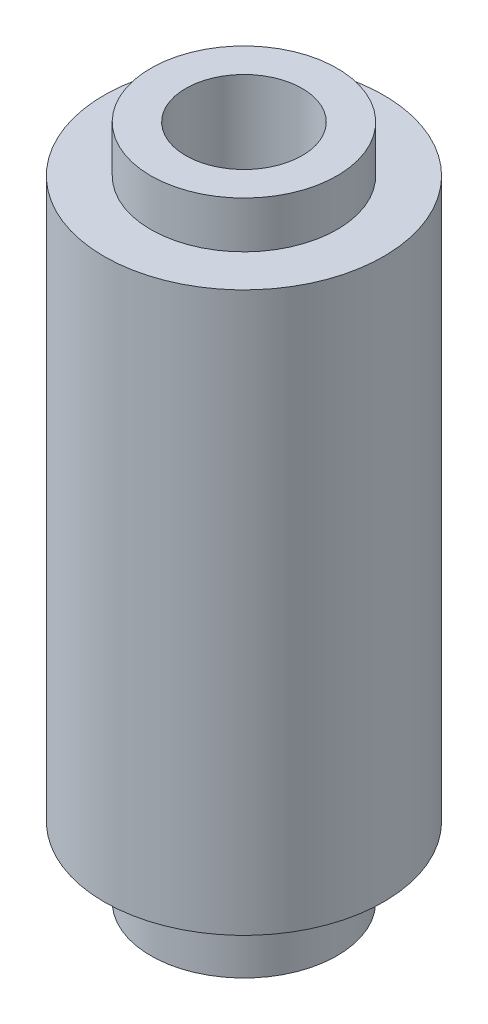
SolidWorks part; units mm, degrees
ref_plane "Front plane" through (0, 0, 0) normal (0, 0, 1) x (1, 0, 0)
ref_plane "Top plane" through (0, 0, 0) normal (0, 1, 0) x (1, 0, 0)
ref_plane "Right plane" through (0, 0, 0) normal (1, 0, 0) x (0, 0, -1)
other "Configuration Table"
sketch "Sketch 2" plane through (0, 0, 0) normal (0, 1, 0) x (1, 0, 0)
  circle A0 centre (0, 0) radius 3
  dimension "D1" = 6
extrude "Boss-Extrude 1" add sketch "Sketch 2" along normal blind 12
sketch "Sketch 3" plane through (0, 12, 0) normal (0, 1, 0) x (1, 0, 0)
  circle A0 centre (0, 0) radius 2
  dimension "D1" = 4
extrude "Boss-Extrude 2" add sketch "Sketch 3" along normal blind 1
sketch "Sketch 4" plane through (0, 0, 0) normal (0, -1, 0) x (-1, 0, 0)
  circle A0 centre (0, 0) radius 2
extrude "Boss-Extrude 3" add sketch "Sketch 4" along normal blind 1.5
sketch "Sketch 5" plane through (0, 13, 0) normal (0, 1, 0) x (1, 0, 0)
  circle A0 centre (0, 0) radius 1.25
  dimension "D1" = 2.5
extrude "Cut-Extrude 1" cut sketch "Sketch 5" against normal blind 6
sketch "Sketch 6" plane through (0, 7, 0) normal (0, 1, 0) x (1, 0, 0)
  circle A0 centre (0, 0) radius 1.5
  dimension "D1" = 3
extrude "Cut-Extrude 2" cut sketch "Sketch 6" against normal blind 2.5
sketch "Sketch 7" plane through (0, -1.5, 0) normal (0, -1, 0) x (-1, 0, 0)
  line L16 (-0.9741, 1.1407) -> (-1.3859, -0.5739)
  line L17 (-1.3859, -0.5739) -> (0.1176, -1.4954)
  line L18 (0.1176, -1.4954) -> (1.4585, -0.3503)
  line L19 (1.4585, -0.3503) -> (0.7839, 1.2789)
  line L20 (0.7839, 1.2789) -> (-0.9741, 1.1407)
  circle A0 centre (0, 0) radius 1.5 construction
  dimension "D1" = 3
extrude "Cut-Extrude 3" cut sketch "Sketch 7" against normal blind 6
ref_plane "Reference plane 2" through (-0.7839, 0, -1.2789) normal (-0.5226, 0, -0.8526) x (-0.8526, 0, 0.5226)
sketch "Sketch 11" plane through (-0.7839, 0, -1.2789) normal (-0.5226, 0, -0.8526) x (-0.8526, 0, 0.5226)
  circle A0 centre (-0.0934, 1.5893) radius 0.5
extrude "Cut-Extrude 8" cut sketch "Sketch 11" against normal up to next and the other way up to next contours A0
